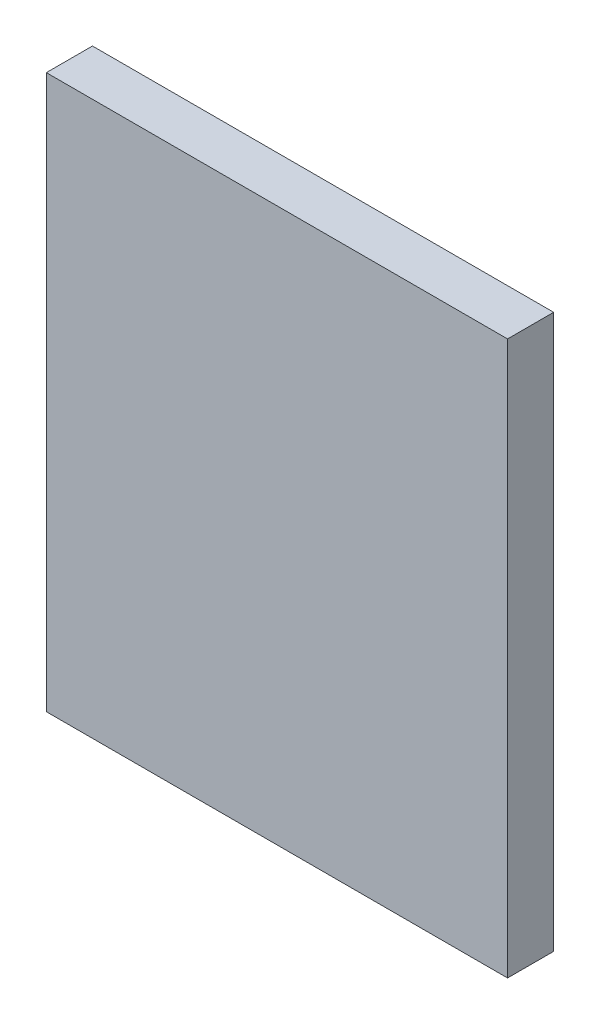
SolidWorks part; units mm, degrees
ref_plane "前视基准面" through (0, 0, 0) normal (0, 0, 1) x (1, 0, 0)
ref_plane "上视基准面" through (0, 0, 0) normal (0, 1, 0) x (1, 0, 0)
ref_plane "右视基准面" through (0, 0, 0) normal (1, 0, 0) x (0, 0, -1)
sketch "草图1" plane through (0, 0, 0) normal (0, 0, 1) x (1, 0, 0)
  line L0 (0, 0) -> (0, 150)
  line L1 (0, 150) -> (50, 150)
  line L2 (50, 150) -> (50, 0)
  line L3 (50, 0) -> (0, 0)
extrude "凸台-拉伸1" add sketch "草图1" along normal blind 10
sketch "草图2" plane through (0, 150, 0) normal (0, 1, 0) x (1, 0, 0)
  line L8 (60, 10) -> (-10, 10)
  line L9 (-10, 10) -> (-10, -20)
  line L10 (-10, -20) -> (60, -20)
  line L11 (60, -20) -> (60, 10)
  line L12 (60, 10) -> (-10, 10)
  line L13 (-10, 10) -> (-10, -20)
  line L14 (-10, -20) -> (60, -20)
  line L15 (60, -20) -> (60, 10)
  dimension "D1" = 10
extrude "切除-拉伸1" cut sketch "草图2" against normal blind 50
sketch "草图3" plane through (0, 0, 0) normal (-1, 0, 0) x (0, 0, 1)
  line L8 (10, 100) -> (0, 100)
  line L9 (0, 100) -> (0, 0)
  line L10 (0, 0) -> (10, 0)
  line L11 (10, 0) -> (10, 100)
  line L12 (10, 100) -> (0, 100)
  line L13 (0, 100) -> (0, 0)
  line L14 (0, 0) -> (10, 0)
  line L15 (10, 0) -> (10, 100)
  dimension "D1" = 0
extrude "凸台-拉伸2" add sketch "草图3" along normal blind 50
sketch "草图4" plane through (0, 0, 0) normal (0, -1, 0) x (1, 0, 0)
  line L8 (-50, 0) -> (50, 0)
  line L9 (50, 0) -> (50, 10)
  line L10 (50, 10) -> (-50, 10)
  line L11 (-50, 10) -> (-50, 0)
  line L12 (-50, 0) -> (50, 0)
  line L13 (50, 0) -> (50, 10)
  line L14 (50, 10) -> (-50, 10)
  line L15 (-50, 10) -> (-50, 0)
  dimension "D1" = 0
extrude "凸台-拉伸3" add sketch "草图4" along normal blind 20
